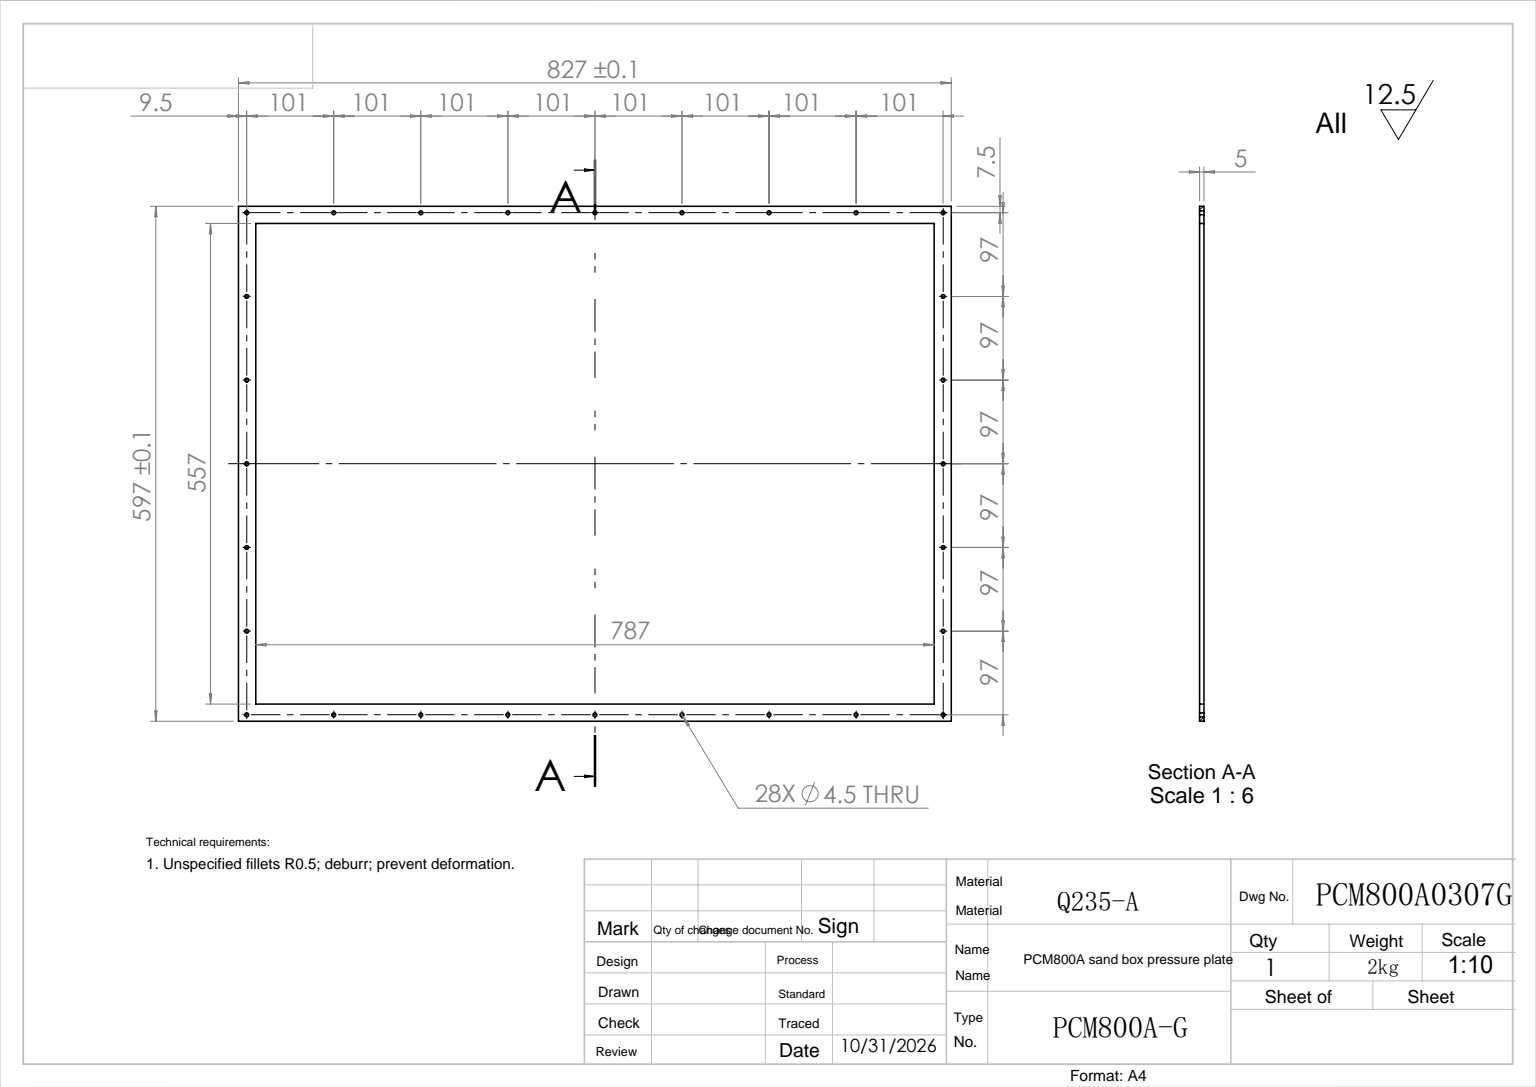
SolidWorks part; units mm, degrees
ref_plane "前视" through (0, 0, 0) normal (0, 0, 1) x (1, 0, 0)
ref_plane "上视" through (0, 0, 0) normal (0, 1, 0) x (1, 0, 0)
ref_plane "右视" through (0, 0, 0) normal (1, 0, 0) x (0, 0, -1)
sketch "草图1" plane through (0, 0, 0) normal (0, 1, 0) x (1, 0, 0)
  line L1 (0, 0) -> (827, 0)
  line L2 (0, 0) -> (0, 597)
  line L3 (0, 597) -> (827, 597)
  line L4 (827, 0) -> (827, 597)
  line L5 (20, 20) -> (807, 20)
  line L6 (20, 20) -> (20, 577)
  line L7 (20, 577) -> (807, 577)
  line L8 (807, 20) -> (807, 577)
  dimension "D1" = 597
  dimension "D2" = 827
  dimension "D3" = 20
  dimension "D4" = 20
  dimension "D5" = 20
  dimension "D6" = 20
extrude "拉伸1" add sketch "草图1" along normal blind 5
sketch "草图2" plane through (0, 5, 0) normal (0, 1, 0) x (-1, 0, 0)
  line L0 (-817.5, -589.5) -> (-817.5, -7.5) construction
  line L1 (-817.5, -7.5) -> (-9.5, -7.5) construction
  line L2 (-9.5, -7.5) -> (-9.5, -589.5) construction
  line L3 (-9.5, -589.5) -> (-817.5, -589.5) construction
  line L4 (-827, 0) -> (-827, -597) construction
  line L5 (-827, -597) -> (0, -597) construction
  line L6 (0, 0) -> (-827, 0) construction
  line L7 (0, -597) -> (0, 0) construction
  circle A0 centre (-817.5, -589.5) radius 2.25
  dimension "D1" = 9.5
  dimension "D2" = 7.5
  dimension "D3" = 7.5
  dimension "D4" = 9.5
extrude "切除-拉伸1" cut sketch "草图2" against normal blind 5
pattern_linear "阵列(线性)1" count 9 spacing 101 along (-1, 0, 0) of "切除-拉伸1"
pattern_linear "阵列(线性)2" count 7 spacing 97 along (0, 0, 1) of "切除-拉伸1"
pattern_linear "阵列(线性)3" count 9 spacing 101 along (-1, 0, 0) of "阵列(线性)2"
